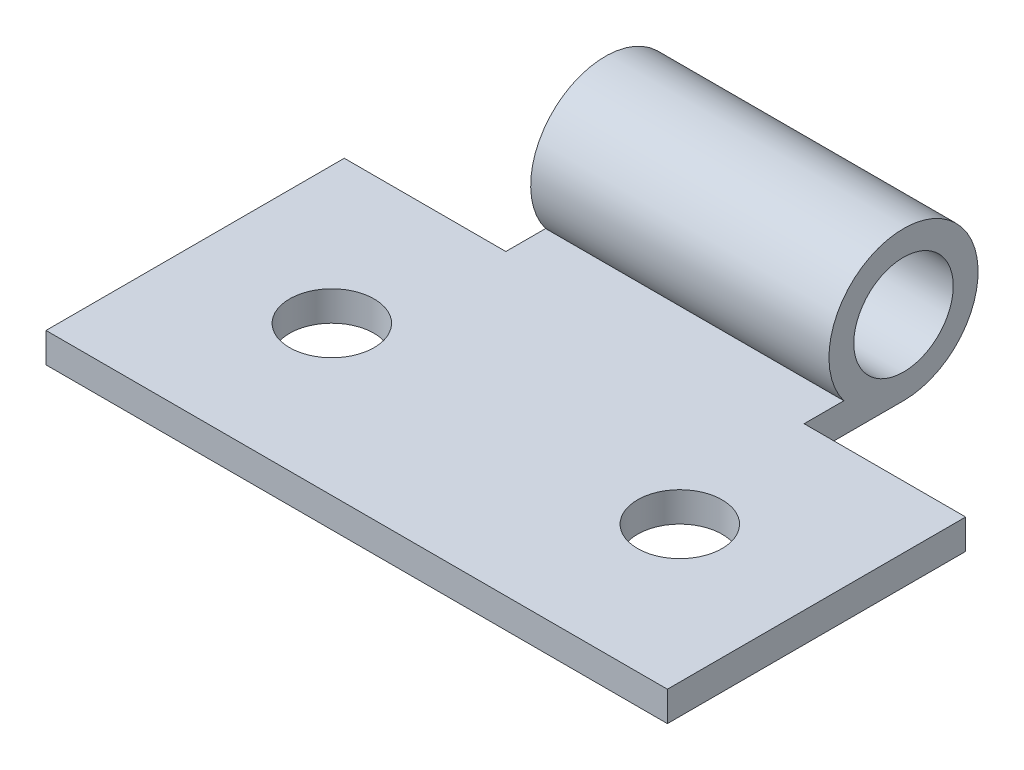
SolidWorks part; units mm, degrees
material "AISI 304"
ref_plane "前视基准面" through (0, 0, 0) normal (0, 0, 1) x (1, 0, 0)
ref_plane "上视基准面" through (0, 0, 0) normal (0, 1, 0) x (1, 0, 0)
ref_plane "右视基准面" through (0, 0, 0) normal (1, 0, 0) x (0, 0, -1)
sketch "草图1" plane through (0, 0, 0) normal (1, 0, 0) x (0, 0, -1)
  line L0 (0, -3) -> (-16, -3)
  line L1 (-16, -3) -> (-16, -1.8)
  line L2 (-16, -1.8) -> (-2.4, -1.8)
  arc A0 (0, -3) -> (-2.4, -1.8) centre (0, 0) ccw
  circle A1 centre (0, 0) radius 2
  dimension "D1" = 3
  dimension "D4" = 4
  dimension "D2" = 16
  dimension "D3" = 1.2
extrude "凸台-拉伸1" add sketch "草图1" along normal mid plane 25
sketch "草图2" plane through (0, -1.8, 0) normal (0, 1, 0) x (1, 0, 0)
  line L0 (-7, -10) -> (7, -10) construction
  line L1 (0, 0) -> (0, -16) construction
  line L2 (12.5, -16) -> (-12.5, -16) construction
  circle A0 centre (-7, -10) radius 1.7
  circle A1 centre (7, -10) radius 1.7
  dimension "D1" = 10
  dimension "D3" = 3.4
  dimension "D2" = 14
extrude "切除-拉伸1" cut sketch "草图2" against normal through all
sketch "草图3" plane through (12.5, 0, 0) normal (1, 0, 0) x (0, 0, -1)
  line L0 (-16, -3) -> (0, -3) construction
  line L1 (-2.4, -1.8) -> (-16, -1.8) construction
  line L2 (-4, -3) -> (0, -3)
  line L3 (-2.4, -1.8) -> (-4, -1.8)
  line L4 (-4, -1.8) -> (-4, -3)
  arc A0 (0, -3) -> (-2.4, -1.8) centre (0, 0) ccw construction
  arc A1 (0, -3) -> (-2.4, -1.8) centre (0, 0) ccw
  dimension "D1" = 4
extrude "切除-拉伸2" cut sketch "草图3" against normal blind 6.5
mirror "镜向1" about plane through (0, 0, 0) normal (1, 0, 0) of "切除-拉伸2"
